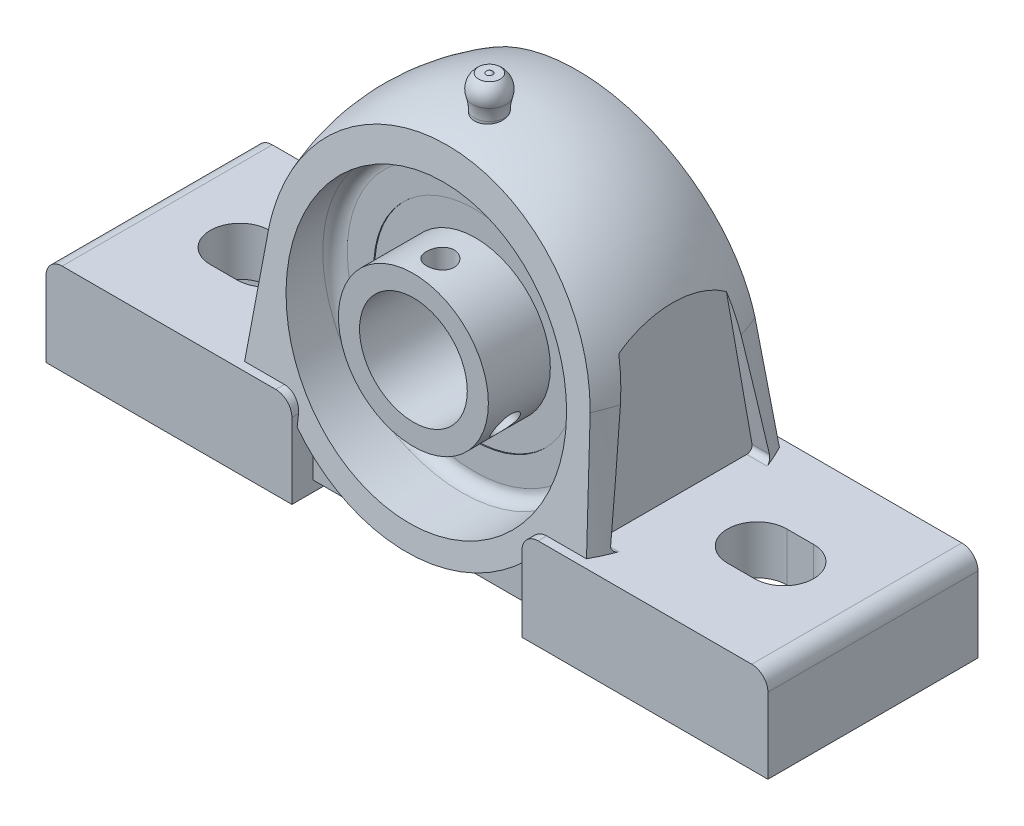
from build123d import *

# Parameters (mm, degrees)
BASE_EXTRUDE_DEPTH              = 84.85
CUT_EXTRUDE1_DEPTH              = 55.135249472
CUT_EXTRUDE1_DEPTH_BACK         = 55.135249472
SKETCH5_OUTSIDE_W               = 60.452
SKETCH5_OUTSIDE_H               = 88.062
BOSS_EXTRUDE4_REACH             = 60.025
BOSS_EXTRUDE4_DIRECTION_2_REACH = 60.025
BOSS_EXTRUDE1_DEPTH             = 19.5
BOSS_EXTRUDE1_DEPTH_BACK        = 19.5
CUT_EXTRUDE3_DEPTH              = 101.761654379
CUT_EXTRUDE4_DEPTH              = 7.99
CUT_EXTRUDE4_DRAFT              = -1
CUT_EXTRUDE4_PROFILE_2_DEPTH    = 7.99
CUT_EXTRUDE4_PROFILE_2_DRAFT    = -1
CIRPATTERN1_COUNT               = 12
SKETCH14_W                      = 31
SKETCH14_H                      = 3.915
SKETCH16_W                      = 2.567
SKETCH16_H                      = 6.115
SKETCH15_W                      = 0.1
SKETCH15_H                      = 5.145
CIRPATTERN2_COUNT               = 2
CIRPATTERN2_ANGLE               = 120
CUT_EXTRUDE5_START              = 29.813111
CUT_EXTRUDE5_DEPTH              = 8.586889
CUT_EXTRUDE6_START              = -38.4
CUT_EXTRUDE6_DEPTH              = 8.49652


with BuildPart() as part:
    # Sketch1 → Base-Extrude (new body)
    with BuildSketch(Plane(origin=(0, -31.3, 0), x_dir=(-1, 0, 0), z_dir=(0, 1, 0))):
        with BuildLine():
            Line((-33.636057661, 18.525), (33.636057661, 18.525))
            ThreePointArc((33.636057661, 18.525), (38.4, 0), (33.636057661, -18.525))
            Line((33.636057661, -18.525), (-33.636057661, -18.525))
            ThreePointArc((-33.636057661, -18.525), (-38.4, 0), (-33.636057661, 18.525))
        make_face()
    extrude(amount=BASE_EXTRUDE_DEPTH)

    # Cut-Sweep1: sweep along a path in Sketch3
    with BuildLine(Plane.XY) as cut_sweep1_path:
        Line((-38.4, -31.3), (-32.994675679, 4.923512654))
        ThreePointArc((-32.994675679, 4.923512654), (0, 33.36), (32.994675679, 4.923512654))
        Line((32.994675679, 4.923512654), (38.4, -31.3))
    # Sketch2 → Cut-Sweep1 (sweep, cut)
    with BuildSketch(Plane(origin=(0, -31.3, 0), x_dir=(-1, 0, 0), z_dir=(0, 1, 0))):
        with BuildLine():
            Line((-33.636057661, 18.525), (-123.25, 18.525))
            Line((-123.25, 18.525), (-123.25, -18.525))
            Line((-123.25, -18.525), (-33.636057661, -18.525))
            ThreePointArc((-33.636057661, -18.525), (-38.4, 0), (-33.636057661, 18.525))
        make_face()
    sweep(path=cut_sweep1_path.line, mode=Mode.SUBTRACT)

    # Sketch5 outside → Cut-Extrude1 (cut, two sides: drawn at the far end of the back side and taken through both)
    with BuildSketch(Plane(origin=(0, 0, 0), x_dir=(0, 0, -1), z_dir=(1, 0, 0)).offset(-CUT_EXTRUDE1_DEPTH_BACK)):
        with Locations((0, 1.03)):
            Rectangle(SKETCH5_OUTSIDE_W, SKETCH5_OUTSIDE_H)
        Polygon((11.7, 34.36), (18.525, -21.38), (15.6, -21.38), (15.6, -34.3), (-15.6, -34.3), (-15.6, -21.38), (-18.525, -21.38), (-11.7, 34.36), align=None, mode=Mode.SUBTRACT)
    extrude(amount=CUT_EXTRUDE1_DEPTH + CUT_EXTRUDE1_DEPTH_BACK, mode=Mode.SUBTRACT)

    # Sketch6 → Cut-Revolve2 (revolve, cut)
    with BuildSketch(Plane(origin=(0, 0, 0), x_dir=(0, 0, -1), z_dir=(1, 0, 0)), mode=Mode.PRIVATE) as cut_revolve2_sk:
        with BuildLine():
            Line((-22.565101692, 25.847619048), (-9.277190476, 25.847619048))
            ThreePointArc((-9.277190476, 25.847619048), (-7.666973648, 25.180645399), (-7, 23.570428571))
            Line((-7, 23.570428571), (-7, 22.433234274))
            ThreePointArc((-7, 22.433234274), (-6.069160332, 22.702759587), (-5.128, 22.933678641))
            Line((-5.128, 22.933678641), (-5.128, 25.847619048))
            Line((-5.128, 25.847619048), (-3.256, 25.847619048))
            Line((-3.256, 25.847619048), (-3.256, 23.273342347))
            ThreePointArc((-3.256, 23.273342347), (1.918548773, 23.421553548), (7, 22.433234274))
            Line((7, 22.433234274), (7, 23.570428571))
            ThreePointArc((7, 23.570428571), (7.666973648, 25.180645399), (9.277190476, 25.847619048))
            Line((9.277190476, 25.847619048), (22.565101692, 25.847619048))
            Line((22.565101692, 25.847619048), (25.729974315, 0))
            Line((25.729974315, 0), (-25.729974315, 0))
            Line((-25.729974315, 0), (-22.565101692, 25.847619048))
        make_face()
    revolve(cut_revolve2_sk.sketch.rotate(Axis((0, 0, 0), (0, 0, -1)), 180), axis=Axis((0, 0, 0), (0, 0, -1)), mode=Mode.SUBTRACT)

    # Sketch11 → Boss-Revolve1 (revolve)
    with BuildSketch(Plane.XY.offset(4.192)):
        with BuildLine():
            Line((0, 31.44046273), (0, 39.36))
            ThreePointArc((0, 39.36), (-0.328456711, 39.290107141), (-0.6, 39.092539267))
            Line((-0.6, 39.092539267), (-2, 39.092539267))
            ThreePointArc((-2, 39.092539267), (-3.100653507, 37.504684437), (-3.105555556, 35.572665525))
            ThreePointArc((-3.105555556, 35.572665525), (-2.83938828, 34.406746373), (-2.75, 33.214176785))
            Line((-2.75, 33.214176785), (-2.75, 31.44046273))
            Line((-2.75, 31.44046273), (0, 31.44046273))
        make_face()
    revolve(axis=Axis((0, 0, 4.192), (0, 1, 0)))

    # Boss-Extrude4: up to this plane
    boss_extrude4_end = Plane(origin=(-38.4, 34.36, -11.7), z_dir=(0, 0.12153581971911598, -0.9925870463214813))
    # Sketch9 → Boss-Extrude4 (add, up to the surface)
    with BuildSketch(Plane.XY, mode=Mode.PRIVATE) as boss_extrude4_sk1:
        with BuildLine():
            Line((14.525667297, -21.38), (21.353177431, -21.38))
            ThreePointArc((21.353177431, -21.38), (0, -30.216925496), (-21.353177431, -21.38))
            Line((-21.353177431, -21.38), (-14.525667297, -21.38))
            ThreePointArc((-14.525667297, -21.38), (0, -25.847619048), (14.525667297, -21.38))
        make_face()
    boss_extrude4_tool1 = split(extrude(boss_extrude4_sk1.sketch, amount=-BOSS_EXTRUDE4_REACH, mode=Mode.PRIVATE), bisect_by=boss_extrude4_end, keep=Keep.BOTH, mode=Mode.PRIVATE)
    add(boss_extrude4_tool1.solids().sort_by_distance((0, -25.877182, 0))[0])

    # Boss-Extrude4 direction 2: up to this plane
    boss_extrude4_direction_2_end = Plane(origin=(-38.4, 34.36, 11.7), z_dir=(0, 0.12153581971911598, 0.9925870463214813))
    # Sketch9 → Boss-Extrude4 direction 2 (add, up to the surface)
    with BuildSketch(Plane.XY, mode=Mode.PRIVATE) as boss_extrude4_direction_2_sk1:
        with BuildLine():
            Line((14.525667297, -21.38), (21.353177431, -21.38))
            ThreePointArc((21.353177431, -21.38), (0, -30.216925496), (-21.353177431, -21.38))
            Line((-21.353177431, -21.38), (-14.525667297, -21.38))
            ThreePointArc((-14.525667297, -21.38), (0, -25.847619048), (14.525667297, -21.38))
        make_face()
    boss_extrude4_direction_2_tool1 = split(extrude(boss_extrude4_direction_2_sk1.sketch, amount=BOSS_EXTRUDE4_DIRECTION_2_REACH, mode=Mode.PRIVATE), bisect_by=boss_extrude4_direction_2_end, keep=Keep.BOTH, mode=Mode.PRIVATE)
    add(boss_extrude4_direction_2_tool1.solids().sort_by_distance((0, -25.877182, 0))[0])

    # Sketch4 → Boss-Extrude1 (add, two sides: drawn at the far end of the back side and taken through both)
    with BuildSketch(Plane.XY.offset(-BOSS_EXTRUDE1_DEPTH_BACK)):
        with BuildLine():
            Line((24.353177431, -16.3), (64, -16.3))
            ThreePointArc((64, -16.3), (66.121320344, -17.178679656), (67, -19.3))
            Line((67, -19.3), (67, -33.3))
            Line((67, -33.3), (21.353177431, -33.3))
            Line((21.353177431, -33.3), (21.353177431, -19.3))
            ThreePointArc((21.353177431, -19.3), (22.231857088, -17.178679656), (24.353177431, -16.3))
        make_face()
        with BuildLine():
            Line((-64, -16.3), (-24.353177431, -16.3))
            ThreePointArc((-24.353177431, -16.3), (-22.231857088, -17.178679656), (-21.353177431, -19.3))
            Line((-21.353177431, -19.3), (-21.353177431, -33.3))
            Line((-21.353177431, -33.3), (-67, -33.3))
            Line((-67, -33.3), (-67, -19.3))
            ThreePointArc((-67, -19.3), (-66.121320344, -17.178679656), (-64, -16.3))
        make_face()
    extrude(amount=BOSS_EXTRUDE1_DEPTH + BOSS_EXTRUDE1_DEPTH_BACK)

    # Sketch7 → Cut-Extrude3 (cut, through all)
    with BuildSketch(Plane.XZ.offset(33.3)):
        with BuildLine():
            Line((-45.5, 5.5), (-50.5, 5.5))
            ThreePointArc((-50.5, 5.5), (-56, 0), (-50.5, -5.5))
            Line((-50.5, -5.5), (-45.5, -5.5))
            ThreePointArc((-45.5, -5.5), (-40, 0), (-45.5, 5.5))
        make_face()
        with BuildLine():
            Line((45.5, -5.5), (50.5, -5.5))
            ThreePointArc((50.5, -5.5), (56, 0), (50.5, 5.5))
            Line((50.5, 5.5), (45.5, 5.5))
            ThreePointArc((45.5, 5.5), (40, 0), (45.5, -5.5))
        make_face()
    extrude(amount=-CUT_EXTRUDE3_DEPTH, mode=Mode.SUBTRACT)


with BuildPart() as cut_extrude4_tool:
    # Sketch10 → Cut-Extrude4 (with draft: the straight prism first)
    with BuildSketch(Plane.XZ.offset(33.3)):
        with BuildLine():
            ThreePointArc((50.5, -10.73), (51.015492065, -9.485492065), (52.26, -8.97))
            Line((52.26, -8.97), (59.975, -8.97))
            ThreePointArc((59.975, -8.97), (61.219507935, -8.454507935), (61.735, -7.21))
            Line((61.735, -7.21), (61.735, 7.21))
            ThreePointArc((61.735, 7.21), (61.219507935, 8.454507935), (59.975, 8.97))
            Line((59.975, 8.97), (52.26, 8.97))
            ThreePointArc((52.26, 8.97), (51.015492065, 9.485492065), (50.5, 10.73))
            Line((50.5, 10.73), (50.5, 12.475))
            ThreePointArc((50.5, 12.475), (49.984507935, 13.719507935), (48.74, 14.235))
            Line((48.74, 14.235), (28.378177431, 14.235))
            ThreePointArc((28.378177431, 14.235), (27.133669496, 13.719507935), (26.618177431, 12.475))
            Line((26.618177431, 12.475), (26.618177431, -12.475))
            ThreePointArc((26.618177431, -12.475), (27.133669496, -13.719507935), (28.378177431, -14.235))
            Line((28.378177431, -14.235), (48.74, -14.235))
            ThreePointArc((48.74, -14.235), (49.984507935, -13.719507935), (50.5, -12.475))
            Line((50.5, -12.475), (50.5, -10.73))
        make_face()
    extrude(amount=-CUT_EXTRUDE4_DEPTH)
    # Cut-Extrude4: the draft: its side faces are tilted about the plane it starts from
    cut_extrude4_sides = [cut_extrude4_tool.faces().sort_by_distance(p)[0] for p in [
        (51.015492065, -29.305, -9.485492065),
        (56.1175, -29.305, -8.97),
        (61.219507935, -29.305, -8.454507935),
        (61.735, -29.305, 0),
        (61.219507935, -29.305, 8.454507935),
        (56.1175, -29.305, 8.97),
        (51.015492065, -29.305, 9.485492065),
        (50.5, -29.305, 11.6025),
        (49.984507935, -29.305, 13.719507935),
        (38.559088716, -29.305, 14.235),
        (27.133669496, -29.305, 13.719507935),
        (26.618177431, -29.305, 0),
        (27.133669496, -29.305, -13.719507935),
        (38.559088716, -29.305, -14.235),
        (49.984507935, -29.305, -13.719507935),
        (50.5, -29.305, -11.6025),
    ]]
    draft(cut_extrude4_sides, Plane.XZ.offset(33.3), CUT_EXTRUDE4_DRAFT)


with BuildPart() as part_1:
    add(part.part)

    # Cut-Extrude4: cut by cut_extrude4_tool
    add(cut_extrude4_tool.part, mode=Mode.SUBTRACT)


with BuildPart() as cut_extrude4_profile_2_tool:
    # Sketch10 → Cut-Extrude4 profile 2 (with draft: the straight prism first)
    with BuildSketch(Plane.XZ.offset(33.3)):
        with BuildLine():
            Line((-59.975, -8.97), (-52.26, -8.97))
            ThreePointArc((-52.26, -8.97), (-51.015492065, -9.485492065), (-50.5, -10.73))
            Line((-50.5, -10.73), (-50.5, -12.475))
            ThreePointArc((-50.5, -12.475), (-49.984507935, -13.719507935), (-48.74, -14.235))
            Line((-48.74, -14.235), (-28.378177431, -14.235))
            ThreePointArc((-28.378177431, -14.235), (-27.133669496, -13.719507935), (-26.618177431, -12.475))
            Line((-26.618177431, -12.475), (-26.618177431, 12.475))
            ThreePointArc((-26.618177431, 12.475), (-27.133669496, 13.719507935), (-28.378177431, 14.235))
            Line((-28.378177431, 14.235), (-48.74, 14.235))
            ThreePointArc((-48.74, 14.235), (-49.984507935, 13.719507935), (-50.5, 12.475))
            Line((-50.5, 12.475), (-50.5, 10.73))
            ThreePointArc((-50.5, 10.73), (-51.015492065, 9.485492065), (-52.26, 8.97))
            Line((-52.26, 8.97), (-59.975, 8.97))
            ThreePointArc((-59.975, 8.97), (-61.219507935, 8.454507935), (-61.735, 7.21))
            Line((-61.735, 7.21), (-61.735, -7.21))
            ThreePointArc((-61.735, -7.21), (-61.219507935, -8.454507935), (-59.975, -8.97))
        make_face()
    extrude(amount=-CUT_EXTRUDE4_PROFILE_2_DEPTH)
    # Cut-Extrude4 profile 2: the draft: its side faces are tilted about the plane it starts from
    cut_extrude4_profile_2_sides = [cut_extrude4_profile_2_tool.faces().sort_by_distance(p)[0] for p in [
        (-49.984507935, -29.305, 13.719507935),
        (-50.5, -29.305, 11.6025),
        (-51.015492065, -29.305, 9.485492065),
        (-56.1175, -29.305, 8.97),
        (-61.219507935, -29.305, 8.454507935),
        (-61.735, -29.305, 0),
        (-61.219507935, -29.305, -8.454507935),
        (-56.1175, -29.305, -8.97),
        (-51.015492065, -29.305, -9.485492065),
        (-50.5, -29.305, -11.6025),
        (-49.984507935, -29.305, -13.719507935),
        (-38.559088716, -29.305, -14.235),
        (-27.133669496, -29.305, -13.719507935),
        (-26.618177431, -29.305, 0),
        (-27.133669496, -29.305, 13.719507935),
        (-38.559088716, -29.305, 14.235),
    ]]
    draft(cut_extrude4_profile_2_sides, Plane.XZ.offset(33.3), CUT_EXTRUDE4_PROFILE_2_DRAFT)


with BuildPart() as part_2:
    add(part_1.part)

    # Cut-Extrude4 profile 2: cut by cut_extrude4_profile_2_tool
    add(cut_extrude4_profile_2_tool.part, mode=Mode.SUBTRACT)

    # Sketch12 → Boss-Revolve3 (revolve)
    with BuildSketch(Plane(origin=(0, 0, 0), x_dir=(0, 0, -1), z_dir=(1, 0, 0)), mode=Mode.PRIVATE) as boss_revolve3_sk:
        with BuildLine():
            Line((7, 22.453234274), (7, 18.66))
            Line((7, 18.66), (-7, 18.66))
            Line((-7, 18.66), (-7, 22.453234274))
            ThreePointArc((-7, 22.453234274), (0, 23.52), (7, 22.453234274))
        make_face()
    revolve(boss_revolve3_sk.sketch.rotate(Axis((0, 0, 0), (0, 0, -1)), 180), axis=Axis((0, 0, 0), (0, 0, -1)))

    # Sketch13 → Boss-Revolve4 (revolve)
    with BuildSketch(Plane(origin=(0, 0, 0), x_dir=(0, 0, -1), z_dir=(1, 0, 0))):
        with BuildLine():
            Line((0, 20.6175), (0, 12.9225))
            ThreePointArc((0, 12.9225), (3.8475, 16.77), (0, 20.6175))
        make_face()
    boss_revolve4 = revolve(axis=Axis((0, 0, 0), (0, 1, 0)))

    # CirPattern1: Boss-Revolve4 ×12 about axis
    cirpattern1_axis = Axis((0, 0, 0), (0, 0, 1))
    for i in range(1, CIRPATTERN1_COUNT):
        add(boss_revolve4.rotate(cirpattern1_axis, i * 360 / CIRPATTERN1_COUNT))

    # Sketch14 → Boss-Revolve5 (revolve)
    with BuildSketch(Plane(origin=(0, 0, 0), x_dir=(0, 0, -1), z_dir=(1, 0, 0)), mode=Mode.PRIVATE) as boss_revolve5_sk:
        with Locations((-2.8, 11.9575)):
            Rectangle(SKETCH14_W, SKETCH14_H)
    revolve(boss_revolve5_sk.sketch.rotate(Axis((0, 0, 0), (0, 0, -1)), 90), axis=Axis((0, 0, 0), (0, 0, -1)))

    # Sketch16 → Cut-Revolve3 (revolve, cut)
    with BuildSketch(Plane(origin=(0, 0, 0), x_dir=(0, 0, -1), z_dir=(1, 0, 0))):
        with Locations((-14.5835, 11.0575)):
            Rectangle(SKETCH16_W, SKETCH16_H)
    cut_revolve3 = revolve(axis=Axis((0, 14.115, 13.3), (0, -1, 0)), mode=Mode.SUBTRACT)

    # Sketch15 → Boss-Revolve6 (revolve)
    with BuildSketch(Plane(origin=(0, 0, 0), x_dir=(0, 0, -1), z_dir=(1, 0, 0)), mode=Mode.PRIVATE) as boss_revolve6_sk:
        with Locations((-6.75, 16.2875)):
            Rectangle(SKETCH15_W, SKETCH15_H)
        with Locations((6.75, 16.2875)):
            Rectangle(SKETCH15_W, SKETCH15_H)
    revolve(boss_revolve6_sk.sketch.rotate(Axis((0, 0, 0), (0, 0, -1)), 180), axis=Axis((0, 0, 0), (0, 0, -1)))

    # CirPattern2: Cut-Revolve3 ×2 about axis
    cirpattern2_axis = Axis((0, 0, -21.702927371), (0, 0, -1))
    for i in range(1, CIRPATTERN2_COUNT):
        add(cut_revolve3.rotate(cirpattern2_axis, i * CIRPATTERN2_ANGLE / (CIRPATTERN2_COUNT - 1)), mode=Mode.SUBTRACT)

    # Sketch 17_2 → Cut-Extrude5 (cut)
    with BuildSketch(Plane(origin=(0, 0, 0), x_dir=(0, 0, -1), z_dir=(1, 0, 0)).offset(CUT_EXTRUDE5_START)):
        with BuildLine():
            Line((6.524492273, 31.44046273), (-6.524492273, 31.44046273))
            Line((-6.524492273, 31.44046273), (-14.735478084, -15.126351822))
            ThreePointArc((-14.735478084, -15.126351822), (-14.516714775, -15.94278761), (-13.750670331, -16.3))
            Line((-13.750670331, -16.3), (13.750670331, -16.3))
            ThreePointArc((13.750670331, -16.3), (14.516714775, -15.94278761), (14.735478084, -15.126351822))
            Line((14.735478084, -15.126351822), (6.524492273, 31.44046273))
        make_face()
    extrude(amount=CUT_EXTRUDE5_DEPTH, mode=Mode.SUBTRACT)

    # Sketch 17_2 2 → Cut-Extrude6 (cut)
    with BuildSketch(Plane(origin=(0, 0, 0), x_dir=(0, 0, -1), z_dir=(1, 0, 0)).offset(CUT_EXTRUDE6_START)):
        with BuildLine():
            Line((6.524492273, 31.44046273), (-6.524492273, 31.44046273))
            Line((-6.524492273, 31.44046273), (-14.735478084, -15.126351822))
            ThreePointArc((-14.735478084, -15.126351822), (-14.516714775, -15.94278761), (-13.750670331, -16.3))
            Line((-13.750670331, -16.3), (13.750670331, -16.3))
            ThreePointArc((13.750670331, -16.3), (14.516714775, -15.94278761), (14.735478084, -15.126351822))
            Line((14.735478084, -15.126351822), (6.524492273, 31.44046273))
        make_face()
    extrude(amount=CUT_EXTRUDE6_DEPTH, mode=Mode.SUBTRACT)


solid = part_2.part
